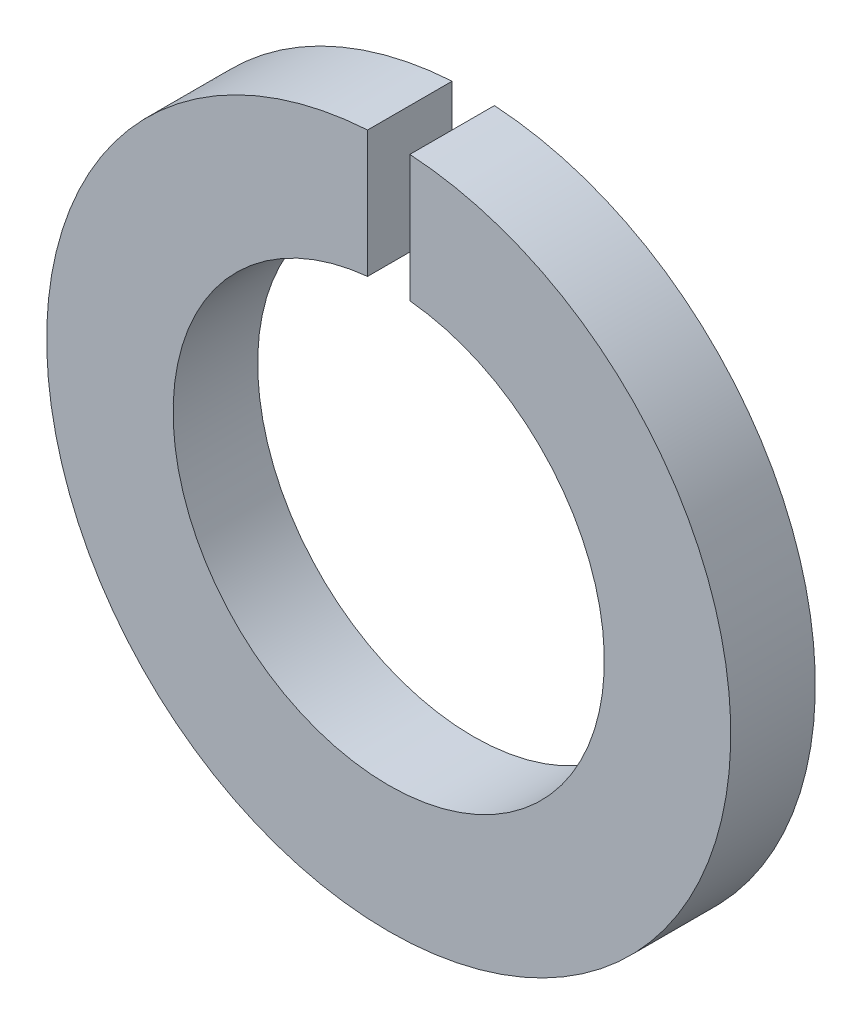
from build123d import *

# Parameters (mm, degrees)
EXTRUDE_1_DEPTH = 2


with BuildPart() as part:
    # Sketch 263 → 拉伸1 (new body)
    with BuildSketch(Plane.XY):
        with BuildLine():
            Line((-0.5, 8.075431016), (-0.5, 5.075431016))
            ThreePointArc((-0.5, 5.075431016), (0, -5.1), (0.5, 5.075431016))
            Line((0.5, 5.075431016), (0.5, 8.075431016))
            ThreePointArc((0.5, 8.075431016), (0, -8.090895259), (-0.5, 8.075431016))
        make_face()
    extrude(amount=EXTRUDE_1_DEPTH)


solid = part.part
